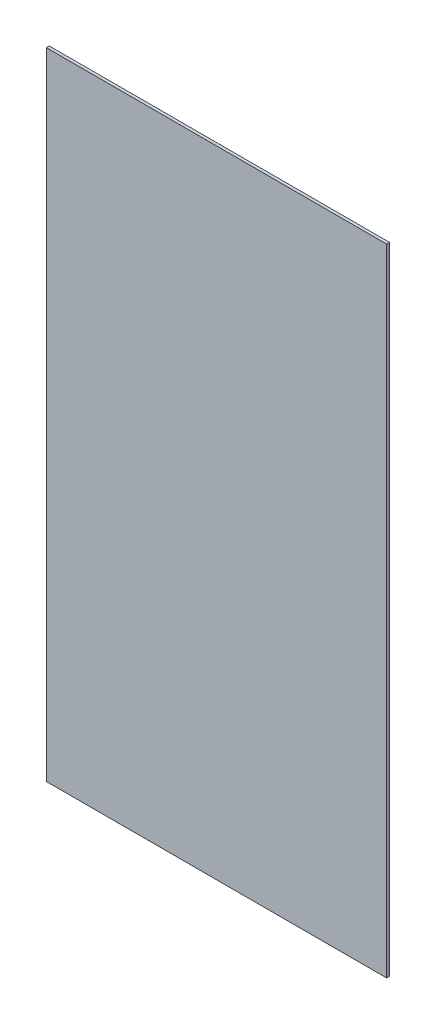
SolidWorks part; units mm, degrees
material "PMMA(有机玻璃)"
ref_plane "前视" through (0, 0, 0) normal (0, 0, 1) x (1, 0, 0)
ref_plane "上视" through (0, 0, 0) normal (0, 1, 0) x (1, 0, 0)
ref_plane "右视" through (0, 0, 0) normal (1, 0, 0) x (0, 0, -1)
sketch "草图1" plane through (0, 0, 0) normal (0, 0, 1) x (1, 0, 0)
  line L1 (-292, 545.5) -> (292, 545.5)
  line L2 (-292, 545.5) -> (-292, -545.5)
  line L3 (-292, -545.5) -> (292, -545.5)
  line L4 (292, 545.5) -> (292, -545.5)
  line L5 (-292, 545.5) -> (292, -545.5) construction
  line L6 (-292, -545.5) -> (292, 545.5) construction
  point P0 (0, 0)
  dimension "D1" = 1091
  dimension "D2" = 584
extrude "凸台-拉伸1" add sketch "草图1" along normal blind 5
hole_wizard "M5 间隙孔1" positions "草图3" profile "草图2" hole size "M5" standard "GB"
sketch "草图3" plane through (0, 0, 5) normal (0, 0, 1) x (1, 0, 0)
  line L0 (-427.5, 273) -> (-427.5, -273) construction
  line L1 (-427.5, -273) -> (427.5, -273) construction
  line L2 (0, 273) -> (0, -273) construction
  line L3 (427.5, 273) -> (-427.5, 273) construction
  line L5 (-427.5, 0) -> (427.5, 0) construction
  line L6 (427.5, -273) -> (427.5, 273) construction
  point P0 (-375, -261)
  point P46 (415.5, 250)
  point P48 (-415.5, 250)
  point P58 (-125, -261)
  point P59 (125, -261)
  point P61 (-125, 261)
  point P62 (125, 261)
  point P64 (-375, 261)
  point P88 (375, -261)
  point P89 (375, 261)
  point P108 (415.5, 0)
  point P109 (-415.5, 0)
  point P110 (415.5, -250)
  point P111 (-415.5, -250)
  dimension "D1" = 12
  dimension "D2" = 12
  dimension "D5" = 3
  dimension "D3" = 12
  dimension "D6" = 4
  dimension "D4" = 2
sketch "草图2" plane through (-375, -261, 5) normal (1, 0, 0) x (0, -1, 0)
  line L0 (0, 0) -> (0, 5)
  line L1 (0, 5) -> (2.75, 5)
  line L2 (2.75, 5) -> (2.75, 0)
  line L5 (2.75, 0) -> (0, 0)
  line L11 (0, -6.35) -> (0, 107.95) construction
  dimension "通孔孔直径" = 5.5
  dimension "通孔孔深度" = 5
